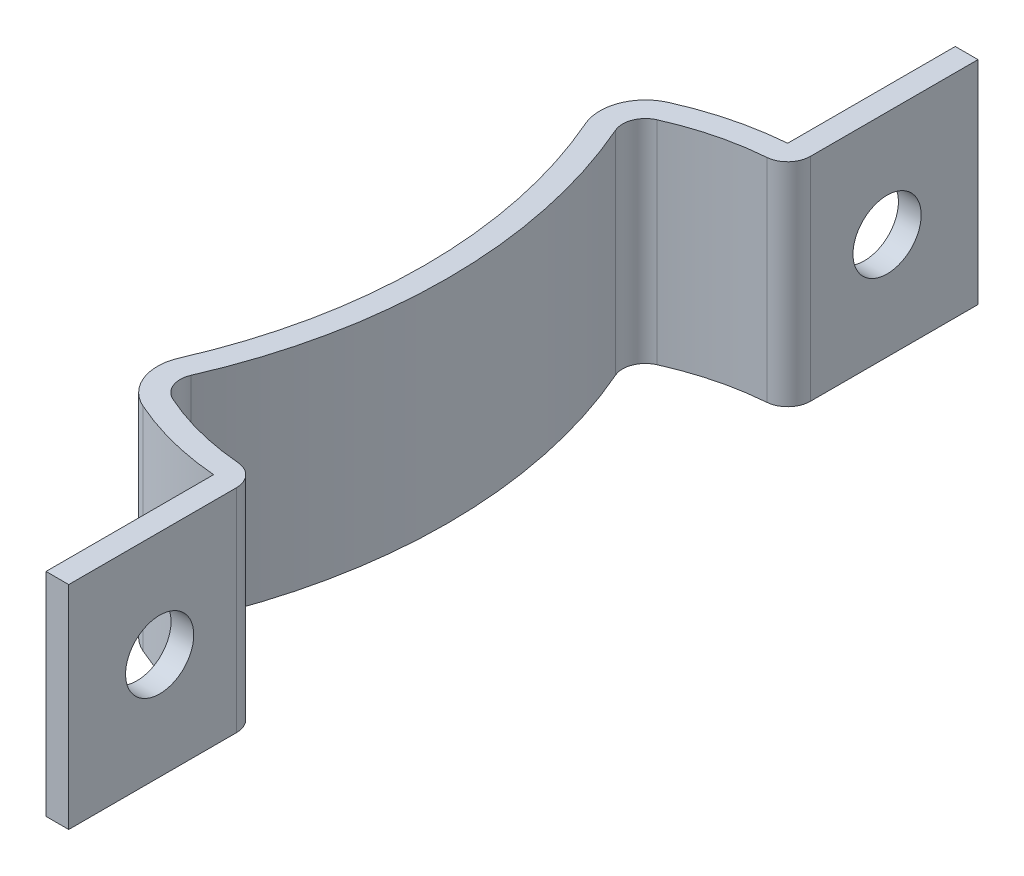
from build123d import *

# Parameters (mm, degrees)
EXTRUDE_THIN3_DEPTH = 14
CUT_EXTRUDE2_REACH  = 36.455
SKETCH3_R           = 2.25


with BuildPart() as part:
    # Sketch1 → Extrude-Thin3 (new body)
    with BuildSketch(Plane(origin=(0, 0, 0), x_dir=(1, 0, 0), z_dir=(0, 1, 0))):
        with BuildLine():
            Line((0, -30), (0, -18.940696925))
            ThreePointArc((0, -18.940696925), (-0.398266916, -17.922765586), (-1.381578947, -17.445378747))
            ThreePointArc((-1.381578947, -17.445378747), (-4.334524238, -16.954701402), (-7.160644531, -15.967941943))
            ThreePointArc((-7.160644531, -15.967941943), (-7.945976251, -15.140108401), (-7.921660959, -13.999291567))
            ThreePointArc((-7.921660959, -13.999291567), (-5, 0), (-7.921660959, 13.999291567))
            ThreePointArc((-7.921660959, 13.999291567), (-7.945976251, 15.140108401), (-7.160644531, 15.967941943))
            ThreePointArc((-7.160644531, 15.967941943), (-4.334524238, 16.954701402), (-1.381578947, 17.445378747))
            ThreePointArc((-1.381578947, 17.445378747), (-0.398266916, 17.922765586), (0, 18.940696925))
            Line((0, 18.940696925), (0, 30))
            Line((0, 30), (-1.5, 30))
            Line((-1.5, 30), (-1.5, 18.940696925))
            ThreePointArc((-1.5, 18.940696925), (-4.706054887, 18.407961522), (-7.774414062, 17.336622681))
            ThreePointArc((-7.774414063, 17.336622681), (-9.345077502, 15.680955597), (-9.296446918, 13.399321928))
            ThreePointArc((-9.296446918, 13.399321928), (-6.5, 0), (-9.296446918, -13.399321928))
            ThreePointArc((-9.296446918, -13.399321928), (-9.345077502, -15.680955597), (-7.774414062, -17.336622681))
            ThreePointArc((-7.774414063, -17.336622681), (-4.706054887, -18.407961522), (-1.5, -18.940696925))
            Line((-1.5, -18.940696925), (-1.5, -30))
            Line((-1.5, -30), (0, -30))
        make_face()
    extrude(amount=EXTRUDE_THIN3_DEPTH)

    # Sketch3 → Cut-Extrude2 (cut, up to next)
    with BuildSketch(Plane(origin=(0, 0, 0), x_dir=(0, 0, -1), z_dir=(1, 0, 0)), mode=Mode.PRIVATE) as cut_extrude2_sk1:
        with Locations((-24, 7)):
            Circle(SKETCH3_R)
    cut_extrude2_tool1 = extrude(cut_extrude2_sk1.sketch, amount=-CUT_EXTRUDE2_REACH, mode=Mode.PRIVATE) & part.part
    # Sketch3 → Cut-Extrude2 (cut, up to next)
    with BuildSketch(Plane(origin=(0, 0, 0), x_dir=(0, 0, -1), z_dir=(1, 0, 0)), mode=Mode.PRIVATE) as cut_extrude2_sk2:
        with Locations((24, 7)):
            Circle(SKETCH3_R)
    cut_extrude2_tool2 = extrude(cut_extrude2_sk2.sketch, amount=-CUT_EXTRUDE2_REACH, mode=Mode.PRIVATE) & part.part
    add(cut_extrude2_tool1.solids().sort_by_distance((0, 7, 24))[0], mode=Mode.SUBTRACT)
    add(cut_extrude2_tool2.solids().sort_by_distance((0, 7, -24))[0], mode=Mode.SUBTRACT)


solid = part.part
